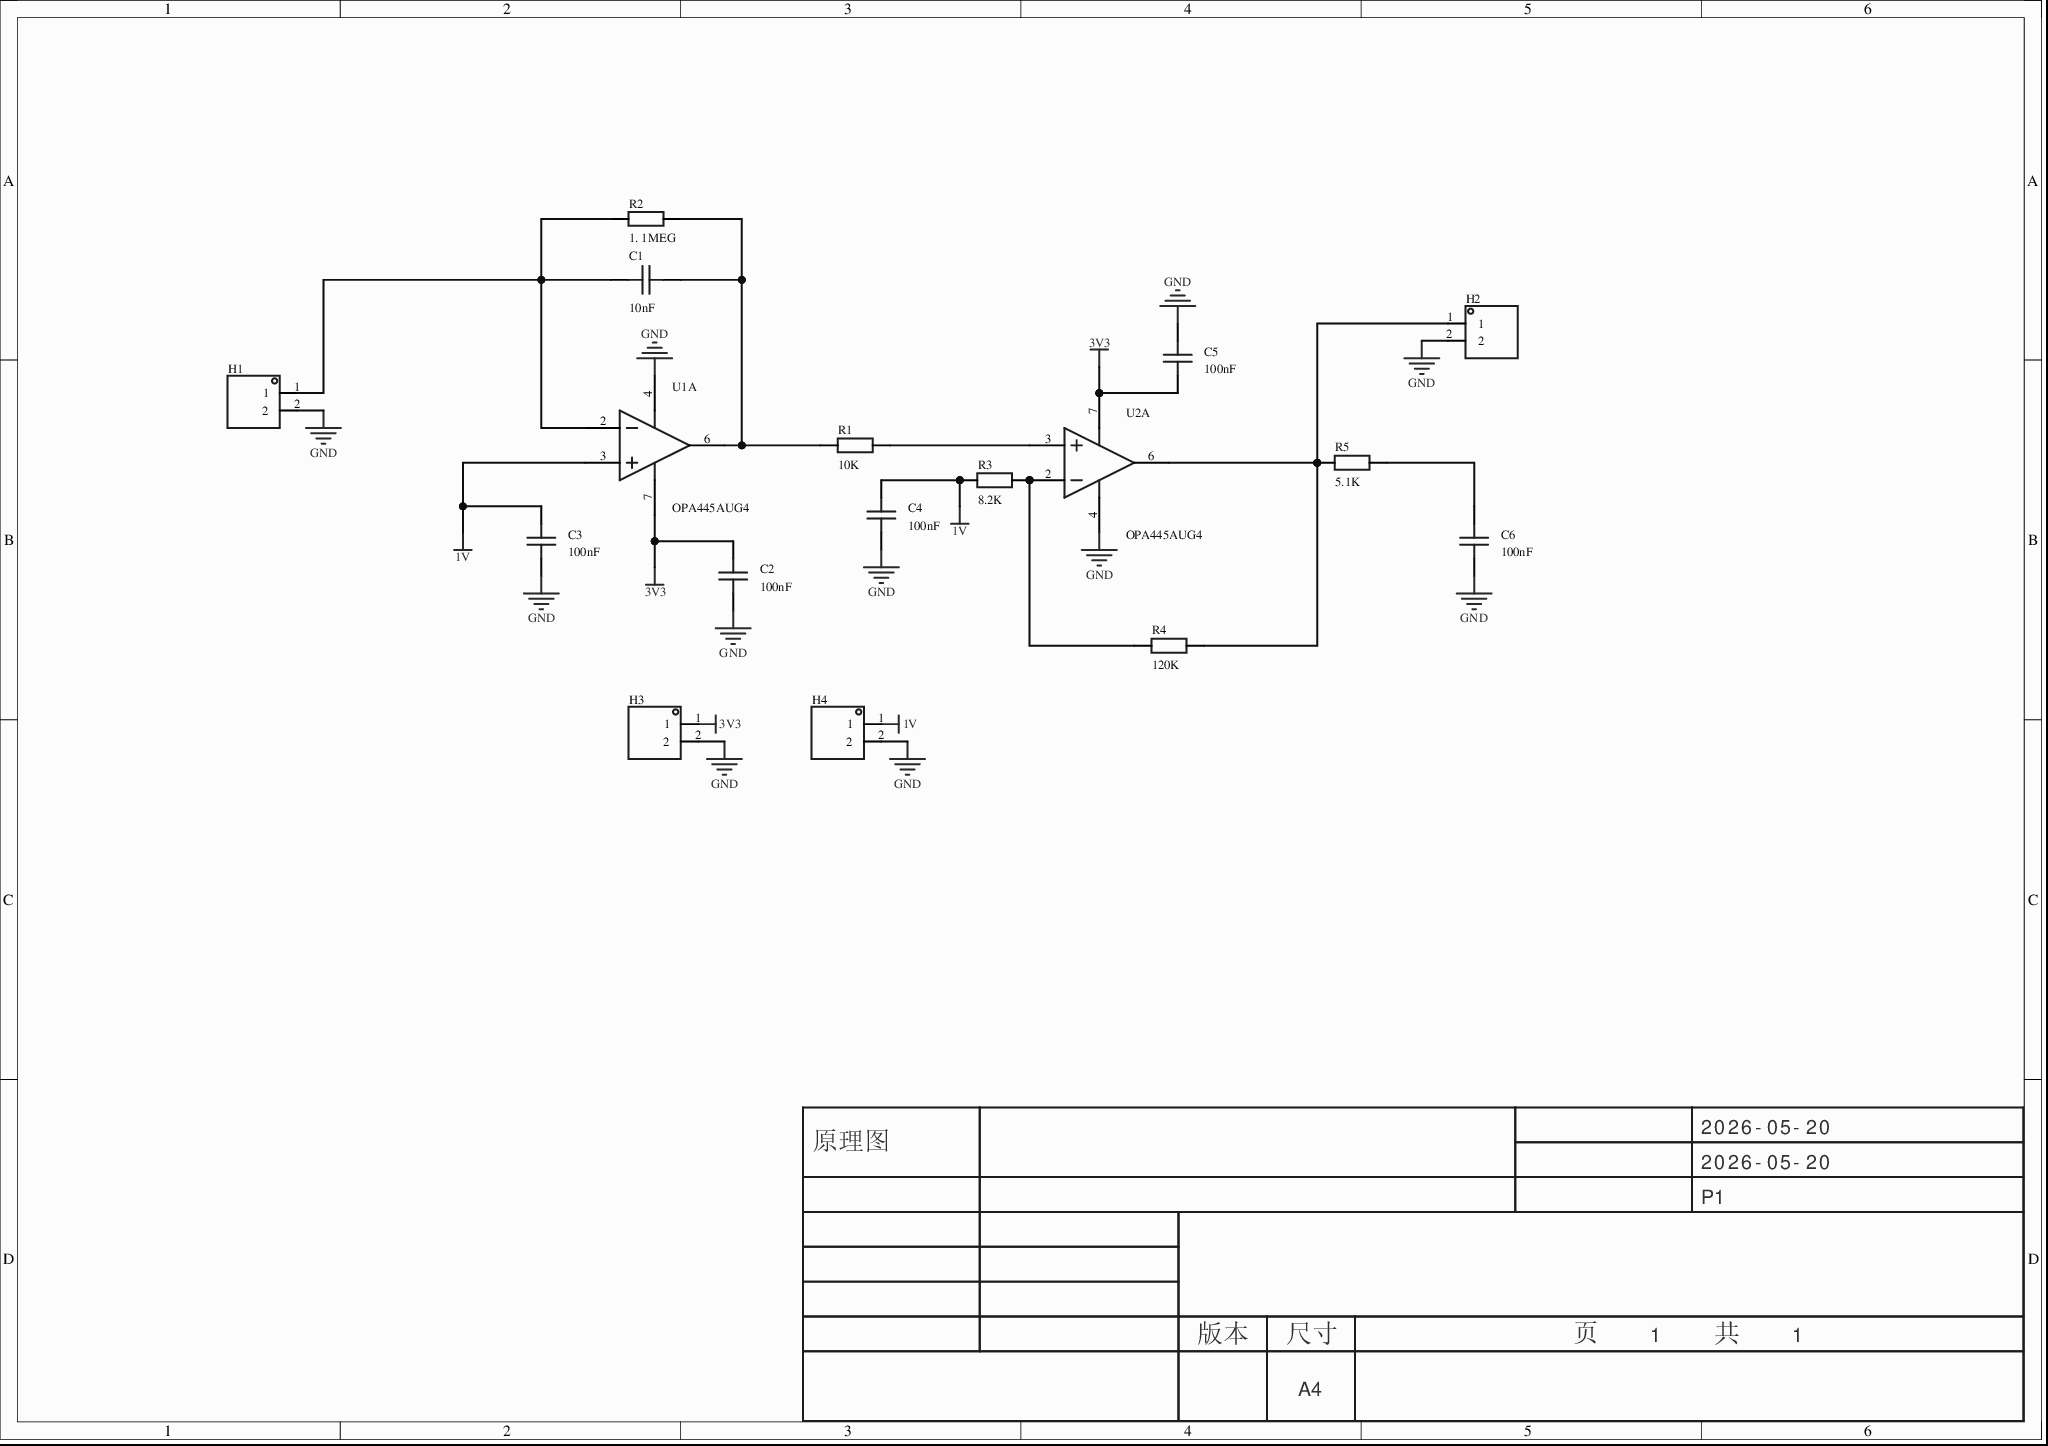
[diagram p0: MISC51758-3.schdoc]
# Altium project MISC51758-2.PrjPcb
1 sheet, 17 parts. Net scope: global (net labels, ports and power ports of the same name join across sheets).
Board file: MISC51758.pcbdoc

## Sheet MISC51758-3.schdoc
size 297 x 209 mm; Version: V1.0; @Project Name: MISC51758; @Update Date: 2026-05-20; @Create Date: 2026-05-20; @Board Name: MISC51758; @Create Time: 00:52:06; @Page Count: 1; @Page No: 1; @Schematic Name: MISC51758; @Update Time: 00:52:06; Size: A4

### Parts
C1  10nF  [C0603]
C2  100nF  [C0603]
C3  100nF  [C0603]
C4  100nF  [C0603]
C5  100nF  [C0603]
C6  100nF  [C0603]
H1  (no value)  [HDR-TH_2P-P2.54-V-M-1]
H2  (no value)  [HDR-TH_2P-P2.54-V-M-1]
H3  (no value)  [HDR-TH_2P-P2.54-V-M-1]
H4  (no value)  [HDR-TH_2P-P2.54-V-M-1]
R1  10K  [R0603]
R2  1. 1MEG  [R0603]
R3  8.2K  [R0603]
R4  120K  [R0603]
R5  5.1K  [R0603]
U1  OPA445AUG4  [SOIC-8_L4.9-W3.9-P1.27-LS6.0-BL]  (part A of 2)
U2  OPA445AUG4  [SOIC-8_L4.9-W3.9-P1.27-LS6.0-BL]  (part A of 2)

### Nets
1V: C3.2 C4.2 H4.1 R3.1 U1.3(+IN)
3V3: C2.2 C5.2 H3.1 U1.7(VSS) U2.7(VSS)
GND: C2.1 C3.1 C4.1 C5.1 C6.2 H1.2 H2.2 H3.2 H4.2 U1.4(VDD) U2.4(VDD)
NetC1_1: C1.1 H1.1 R2.1 U1.2(-IN)
NetC1_2: C1.2 R1.1 R2.2 U1.6(OUT)
NetC6_1: C6.1 R5.2
NetH2_1: H2.1 R4.2 R5.1 U2.6(OUT)
NetR1_2: R1.2 U2.3(+IN)
NetR3_2: R3.2 R4.1 U2.2(-IN)

### Notes on the sheet
- 2026-05-20
- 原理图
- P1
- 版本
- 尺寸
- A4
- 页    1    共    1

### Library data of the parts
C1-C6 = CAP_0603: Symbol: Capacitance; ConvertToPcb: yes; ModelId: ac125912035d415993ca9572d50418b10819f05c4eef4c71ace90d822a990e87; ModelName: C0603_L1.6-W0.8-H0.8; ModelTransform: 62.992,31.496,0,0,0,0,0,0,0; Device: CAP_0603; AddInBom: yes; Supplier Footprint: 0603; FootprintName: C0603
  C1: Value: 10nF
  C2-C6: Value: 100nF
H1-H4 = HDR-M_2.54_1x2P: Symbol: 210S-1*2P L=11.6MMGold-plated black; ConvertToPcb: yes; ModelId: 79b2e9f2d70a4d68a1b7098f27c6d4c50819f05c4eef4c71ace90d822a990e87; ModelName: HDR-M-2.54_1x2; ModelTransform: 200,100,0,0,0,0,0,0,-118.11; Device: HDR-M_2.54_1x2P; AddInBom: yes; SupplierPart: C124375; Supplier Footprint: 插件; FootprintName: HDR-TH_2P-P2.54-V-M-1
R1-R5 = Res_0603: Symbol: 电阻; ConvertToPcb: yes; ModelId: fc143cca1e79419f9cd78b61e9279f080819f05c4eef4c71ace90d822a990e87; ModelTransform: 31.8897,63.7794,0,90,0,0,0,0,0; Device: Res_0603; AddInBom: yes; Supplier Footprint: 0603; FootprintName: R0603; ModelName: R0603
  R1: Value: 10K
  R2: Value: 1. 1MEG
  R3: Value: 8.2K
  R4: Value: 120K
  R5: Value: 5.1K
U1 U2 = OPA445AUG4: Relevance: []; AddInBom: yes; ModelId: e81d2f7d937b4a6ab1dca543ff5d56a40819f05c4eef4c71ace90d822a990e87; ModelName: SOIC-8_L4.9-W3.9-H1.7-LS6.0-P1.27; ModelTransform: 192.913,236.22,0,0,0,0,0,0,0; Symbol: OPA445AUG4; Device: OPA445AUG4; LCSC Part Name: OPA445AUG4; SupplierPart: C6346558; ManufacturerPart: OPA445AUG4; Supplier Footprint: SOIC-8; JLCPCB Part Class: Extended Part; Supplier: LCSC; ConvertToPcb: yes; FootprintName: SOIC-8_L4.9-W3.9-P1.27-LS6.0-BL